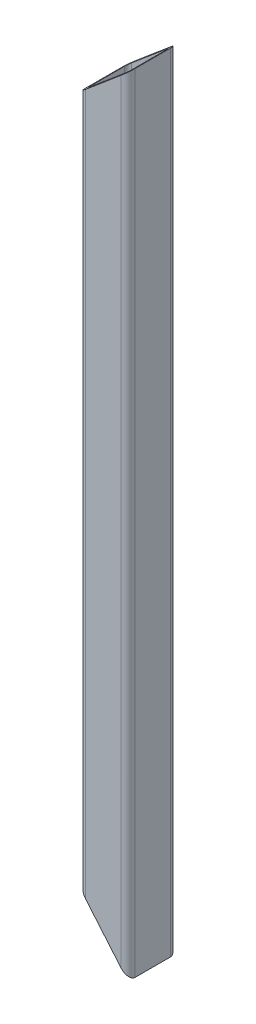
from build123d import *

# Parameters (mm, degrees)
GB_T6728_2002_70_70_5_1_DEPTH = 1116
CUT_EXTRUDE_1_DEPTH           = 1119.740810018
CUT_EXTRUDE_1_DEPTH_BACK      = 1119.740810018


with BuildPart() as part:
    # Sketch1 → 结构用冷弯空心方钢(gb t6728-2002) 70×70×5(1) (new body)
    with BuildSketch(Plane(origin=(0, 0, 0), x_dir=(-1, 0, 0), z_dir=(0, 1, 0))):
        with BuildLine():
            Line((-25, -35), (25, -35))
            ThreePointArc((25, -35), (32.071067812, -32.071067812), (35, -25))
            Line((35, -25), (35, 25))
            ThreePointArc((35, 25), (32.071067812, 32.071067812), (25, 35))
            Line((25, 35), (-25, 35))
            ThreePointArc((-25, 35), (-32.071067812, 32.071067812), (-35, 25))
            Line((-35, 25), (-35, -25))
            ThreePointArc((-35, -25), (-32.071067812, -32.071067812), (-25, -35))
        make_face()
        with BuildLine():
            Line((-25, -30), (25, -30))
            ThreePointArc((25, -30), (28.535533906, -28.535533906), (30, -25))
            Line((30, -25), (30, 25))
            ThreePointArc((30, 25), (28.535533906, 28.535533906), (25, 30))
            Line((25, 30), (-25, 30))
            ThreePointArc((-25, 30), (-28.535533906, 28.535533906), (-30, 25))
            Line((-30, 25), (-30, -25))
            ThreePointArc((-30, -25), (-28.535533906, -28.535533906), (-25, -30))
        make_face(mode=Mode.SUBTRACT)
    extrude(amount=GB_T6728_2002_70_70_5_1_DEPTH)

    # 草图2 → 切除-拉伸1 (cut, two sides: drawn at the far end of the back side and taken through both)
    with BuildSketch(Plane.XY.offset(35).offset(-CUT_EXTRUDE_1_DEPTH_BACK)):
        Polygon((35, 1116), (-35, 1056.963855422), (-35, 1116), align=None)
        Polygon((-35, 83), (35, 0), (-35, 0), align=None)
    extrude(amount=CUT_EXTRUDE_1_DEPTH + CUT_EXTRUDE_1_DEPTH_BACK, mode=Mode.SUBTRACT)


solid = part.part
